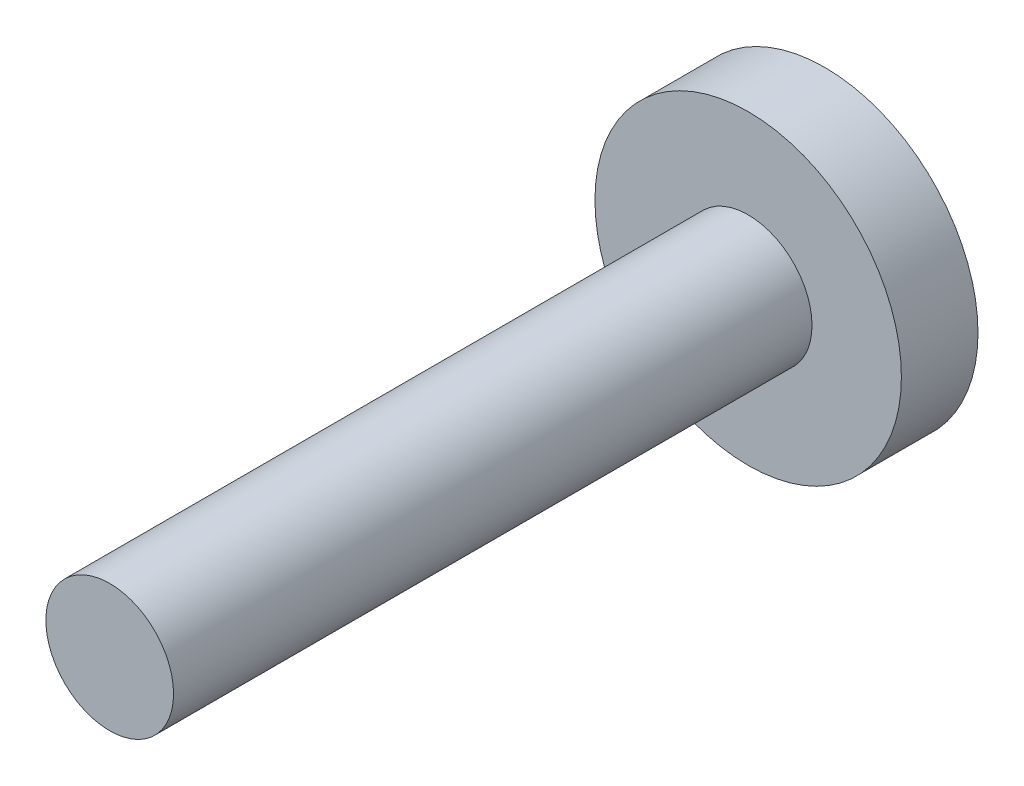
from build123d import *

# Parameters (mm, degrees)
SKETCH_1_R      = 5
EXTRUDE_1_DEPTH = 50
SKETCH_2_R      = 12
EXTRUDE_2_DEPTH = 6


with BuildPart() as part:
    # 草图1 → 凸台-拉伸1 (new body)
    with BuildSketch(Plane.XY):
        Circle(SKETCH_1_R)
    extrude(amount=EXTRUDE_1_DEPTH)

    # 草图2 → 凸台-拉伸2 (add)
    with BuildSketch(Plane.XY):
        Circle(SKETCH_2_R)
    extrude(amount=-EXTRUDE_2_DEPTH)


solid = part.part
